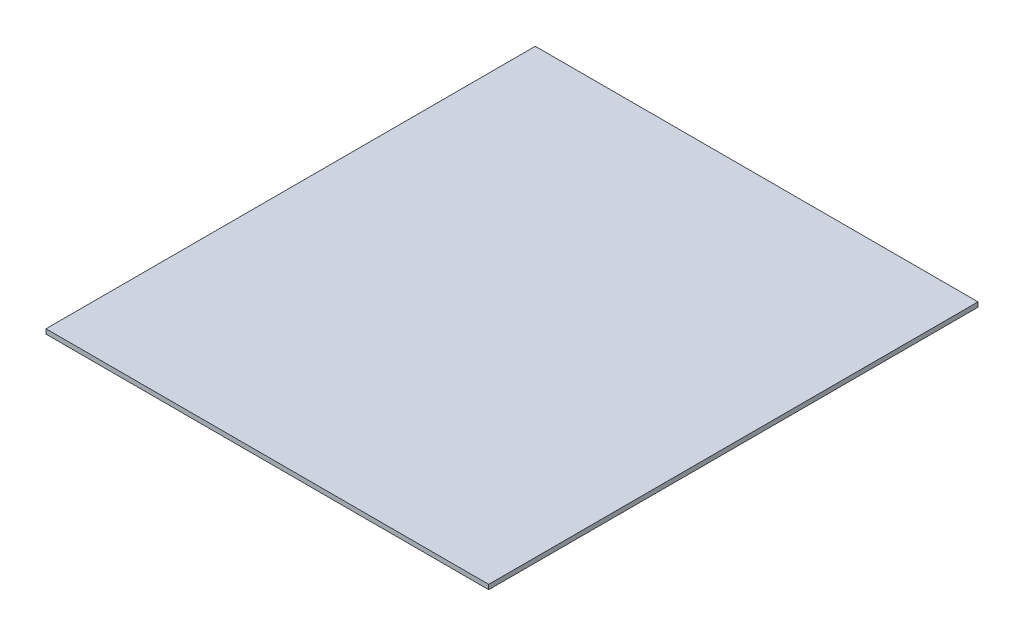
from build123d import *

# Parameters (mm, degrees)
SKETCH1_W           = 380
SKETCH1_H           = 420
BOSS_EXTRUDE1_DEPTH = 4


with BuildPart() as part:
    # Sketch1 → Boss-Extrude1 (new body)
    with BuildSketch(Plane(origin=(0, 0, 0), x_dir=(1, 0, 0), z_dir=(0, 1, 0))):
        Rectangle(SKETCH1_W, SKETCH1_H)
    extrude(amount=BOSS_EXTRUDE1_DEPTH)


solid = part.part
